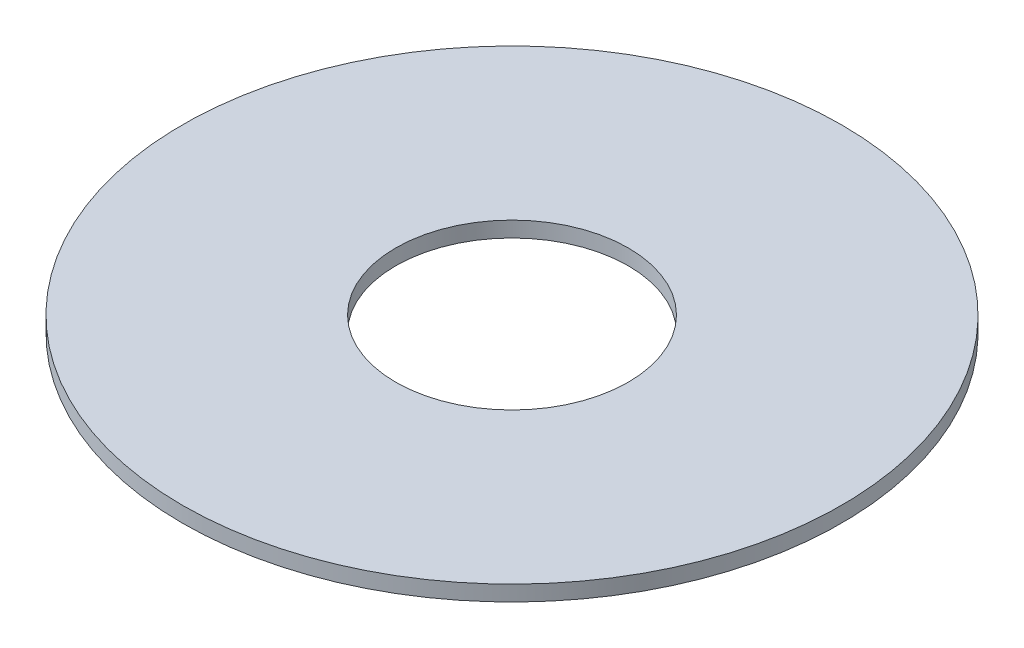
SolidWorks part; units mm, degrees
material "HT200"
ref_plane "Front Plane" through (0, 0, 0) normal (0, 0, 1) x (1, 0, 0)
ref_plane "Top Plane" through (0, 0, 0) normal (0, 1, 0) x (1, 0, 0)
ref_plane "Right Plane" through (0, 0, 0) normal (1, 0, 0) x (0, 0, -1)
other "Configuration Table"
sketch "Sketch1" plane through (0, 0, 0) normal (0, 1, 0) x (1, 0, 0)
  circle A0 centre (0, 0) radius 42.5
  circle A1 centre (0, 0) radius 15
  dimension "D1" = 85
  dimension "D2" = 30
extrude "Boss-Extrude1" add sketch "Sketch1" along normal blind 2
